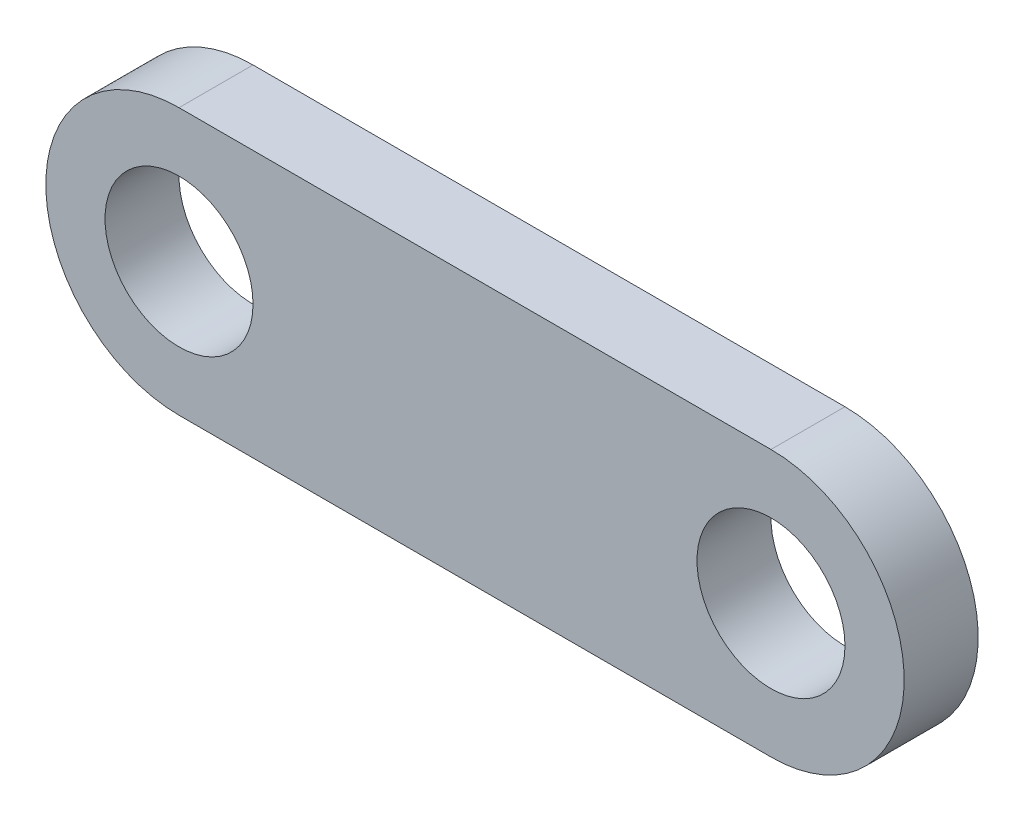
from build123d import *

# Parameters (mm, degrees)
BASE_EXTRUDE_DEPTH = 5
SKETCH2_R          = 5
CUT_EXTRUDE1_DEPTH = 51.069951068


with BuildPart() as part:
    # Sketch1 → Base-Extrude (new body)
    with BuildSketch(Plane.XY):
        with BuildLine():
            Line((0, 9), (40, 9))
            ThreePointArc((40, 9), (49, 0), (40, -9))
            Line((40, -9), (0, -9))
            ThreePointArc((0, -9), (-9, 0), (0, 9))
        make_face()
    extrude(amount=BASE_EXTRUDE_DEPTH)

    # Sketch2 → Cut-Extrude1 (cut, through all)
    with BuildSketch(Plane.XY.offset(5)):
        Circle(SKETCH2_R)
        with Locations((40, 0)):
            Circle(SKETCH2_R)
    extrude(amount=-CUT_EXTRUDE1_DEPTH, mode=Mode.SUBTRACT)


solid = part.part
